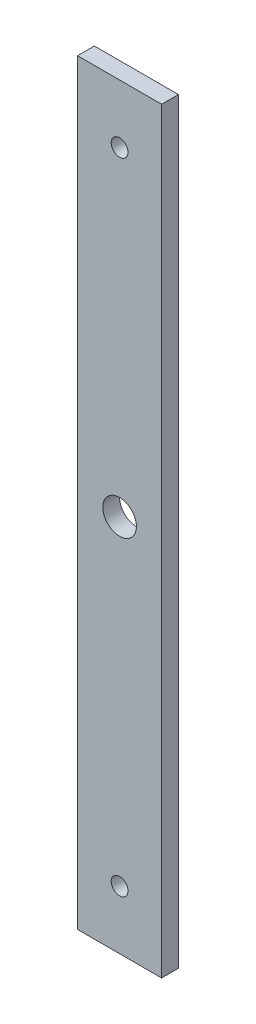
from build123d import *

# Parameters (mm, degrees)
SKETCH_1_W      = 50
SKETCH_1_H      = 450
SKETCH_1_R      = 10
SKETCH_1_R_2    = 5
EXTRUDE_1_DEPTH = 10


with BuildPart() as part:
    # 草图1 → 凸台-拉伸1 (new body)
    with BuildSketch(Plane.XY):
        with Locations((25, 225)):
            Rectangle(SKETCH_1_W, SKETCH_1_H)
        with Locations((25, 225)):
            Circle(SKETCH_1_R, mode=Mode.SUBTRACT)
        with Locations((25, 415.201191985)):
            Circle(SKETCH_1_R_2, mode=Mode.SUBTRACT)
        with Locations(Location((25, 34.798808015, 0), (0, 0, 180))):
            Circle(SKETCH_1_R_2, mode=Mode.SUBTRACT)
    extrude(amount=EXTRUDE_1_DEPTH)


solid = part.part
